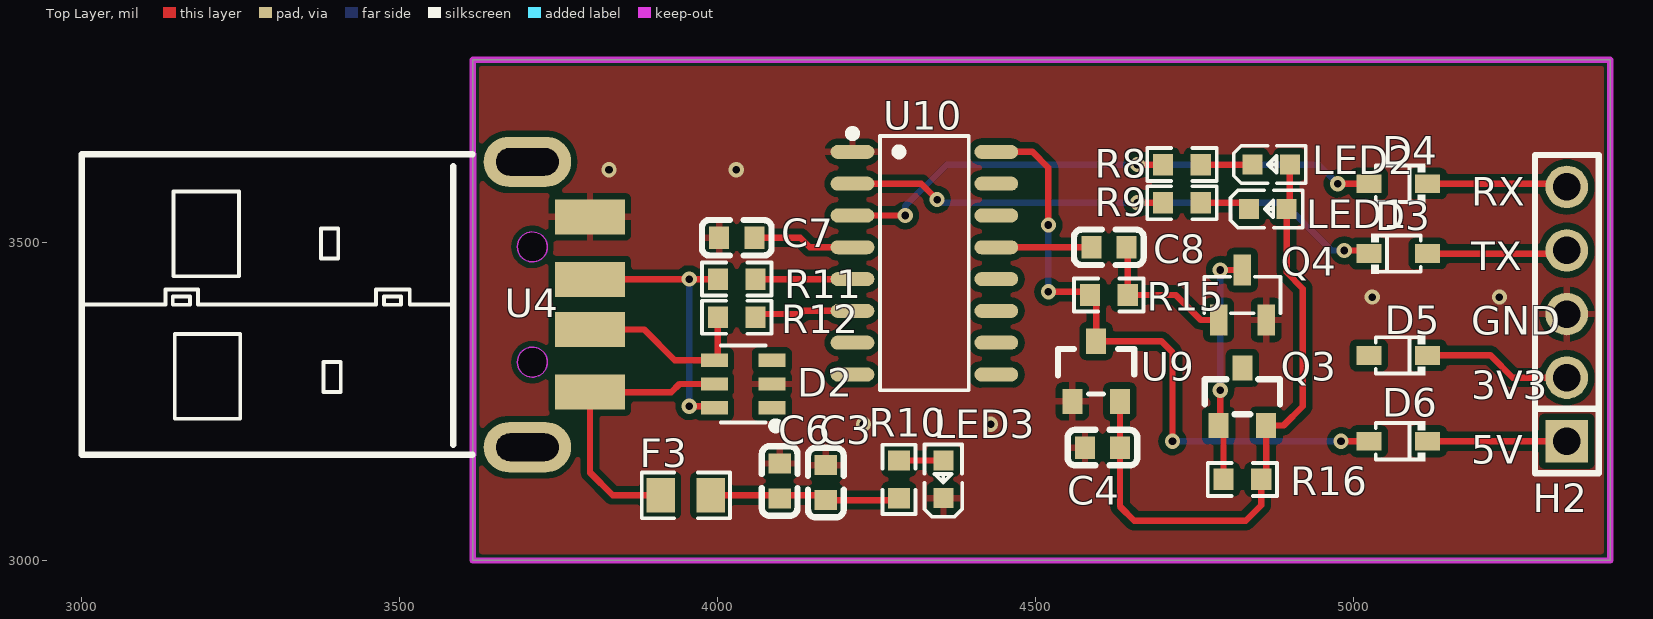
[diagram p0: Top Layer view]
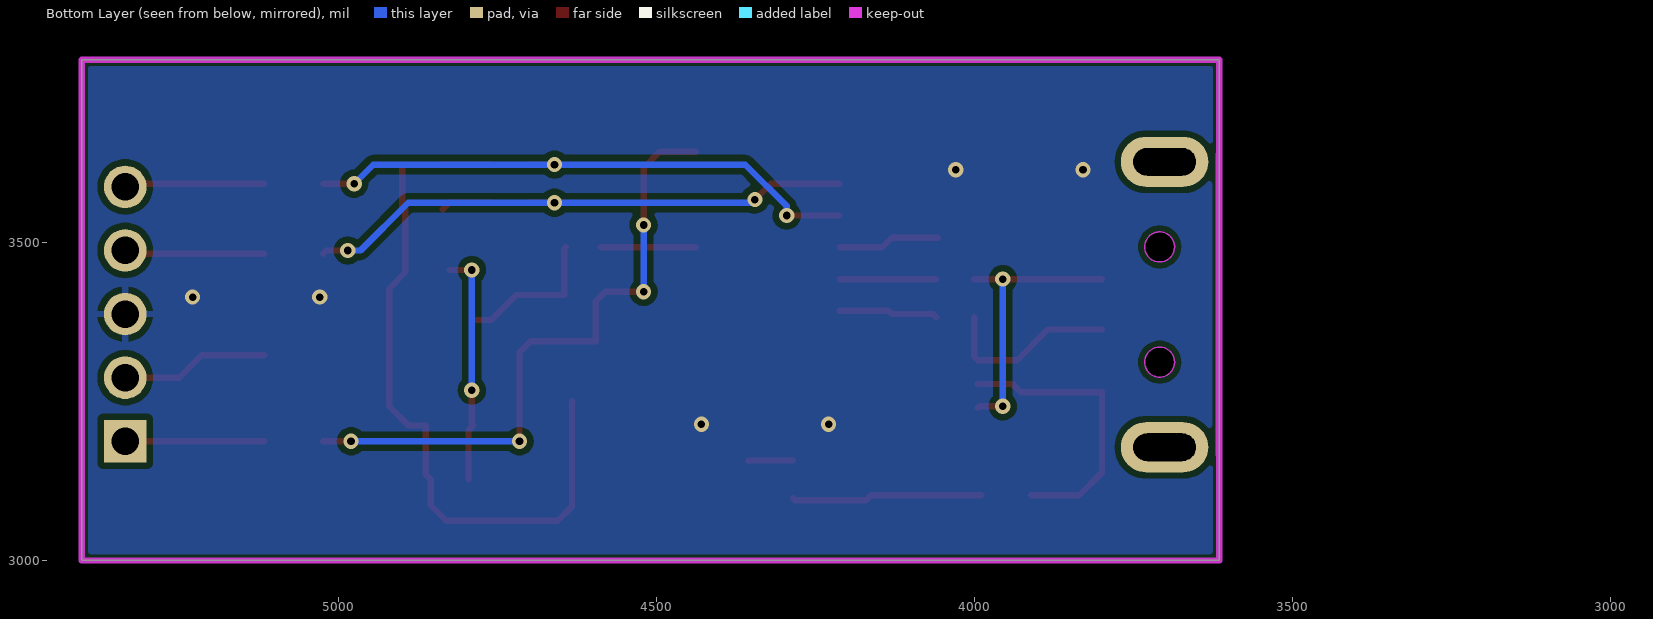
[diagram p1: Bottom Layer view, seen from below]
# Altium PCB MISC51088.pcbdoc
Units mil, origin at the board's own origin, x right, y up, seen from the top; angles counter-clockwise.
Board outline 1788.5 x 787.4 mil, 2 copper layers (Top Layer, Bottom Layer), stack 62.206 mil thick; 27 components, 24 nets, 82 pads, 20 vias.

## Layer stack, top to bottom
Top Solder Mask Layer: solder mask 0.394, Dk 3.3
Top Layer: signal copper 1.379
Dielectric1: surface 59.449, FR4, Dk 4.5
Bottom Layer: signal copper 1.378
Bottom Solder Mask Layer: solder mask 0.394, Dk 3.3

## Board outline
3615.01,3787.4 3615.01,3000 5403.51,3000 5403.51,3787.4

## Design rules (kind name [scope] priority, off if disabled: settings)
BoardOutlineClearance copperThickness2oz_1 [All] p2 off: genericclearance=7.99 ignorepadtopadclearanceinfootprint=FALSE except(0: Arc-SplitContinuation Track-SplitContinuation SMDPad-SplitContinuation THPad-SplitContinuation Via-SplitContinuation Fill-SplitContinuation Region-SplitContinuation Poly-SplitContinuation Text-SplitContinuation Hole-SplitContinuation; 5.98: Arc-CutoutEdge SMDPad-CutoutEdge THPad-CutoutEdge Via-CutoutEdge Fill-CutoutEdge Region-CutoutEdge Text-CutoutEdge; 6.93: Hole-OutlineEdge Hole-CutoutEdge; 10: Poly-OutlineEdge Poly-CutoutEdge; 11.81: Arc-OutlineEdge Track-OutlineEdge SMDPad-OutlineEdge THPad-OutlineEdge Via-OutlineEdge Fill-OutlineEdge Region-OutlineEdge Text-OutlineEdge Track-CutoutEdge)
BoardOutlineClearance Plane_innerPlane_1 [All] p4 off: genericclearance=4.02 ignorepadtopadclearanceinfootprint=FALSE except(0: Arc-SplitContinuation Track-SplitContinuation SMDPad-SplitContinuation THPad-SplitContinuation Via-SplitContinuation Fill-SplitContinuation Region-SplitContinuation Poly-SplitContinuation Text-SplitContinuation Hole-SplitContinuation; 6: SMDPad-CutoutEdge THPad-CutoutEdge Via-CutoutEdge Fill-CutoutEdge Region-CutoutEdge Text-CutoutEdge; 6.93: Hole-OutlineEdge Hole-CutoutEdge; 10: Poly-OutlineEdge Poly-CutoutEdge; 11.8: Arc-OutlineEdge Track-OutlineEdge SMDPad-OutlineEdge THPad-OutlineEdge Via-OutlineEdge Fill-OutlineEdge Region-OutlineEdge Text-OutlineEdge; 11.81: Arc-CutoutEdge Track-CutoutEdge)
BoardOutlineClearance Copper_copperRegion_1 [All] p6 off: genericclearance=4.02 ignorepadtopadclearanceinfootprint=FALSE except(0: Arc-SplitContinuation Track-SplitContinuation SMDPad-SplitContinuation THPad-SplitContinuation Via-SplitContinuation Fill-SplitContinuation Region-SplitContinuation Poly-SplitContinuation Text-SplitContinuation Hole-SplitContinuation; 6: SMDPad-CutoutEdge THPad-CutoutEdge Via-CutoutEdge Fill-CutoutEdge Region-CutoutEdge Text-CutoutEdge; 6.93: Hole-OutlineEdge Hole-CutoutEdge; 10: Poly-OutlineEdge Poly-CutoutEdge; 11.8: Arc-OutlineEdge Track-OutlineEdge SMDPad-OutlineEdge THPad-OutlineEdge Via-OutlineEdge Fill-OutlineEdge Region-OutlineEdge Text-OutlineEdge; 11.81: Arc-CutoutEdge Track-CutoutEdge)
BoardOutlineClearance Copper_copperRegion_copperThickness1oz_1 [All] p8 off: genericclearance=4.02 ignorepadtopadclearanceinfootprint=FALSE except(0: Arc-SplitContinuation Track-SplitContinuation SMDPad-SplitContinuation THPad-SplitContinuation Via-SplitContinuation Fill-SplitContinuation Region-SplitContinuation Poly-SplitContinuation Text-SplitContinuation Hole-SplitContinuation; 6: SMDPad-CutoutEdge THPad-CutoutEdge Via-CutoutEdge Fill-CutoutEdge Region-CutoutEdge Text-CutoutEdge; 6.93: Hole-OutlineEdge Hole-CutoutEdge; 10: Poly-OutlineEdge Poly-CutoutEdge; 11.8: Arc-OutlineEdge Track-OutlineEdge SMDPad-OutlineEdge THPad-OutlineEdge Via-OutlineEdge Fill-OutlineEdge Region-OutlineEdge Text-OutlineEdge; 11.81: Arc-CutoutEdge Track-CutoutEdge)
BoardOutlineClearance Copper_copperRegion_Copper_copperRegion_1 [All] p10 off: genericclearance=4.02 ignorepadtopadclearanceinfootprint=FALSE except(0: Arc-SplitContinuation Track-SplitContinuation SMDPad-SplitContinuation THPad-SplitContinuation Via-SplitContinuation Fill-SplitContinuation Region-SplitContinuation Poly-SplitContinuation Text-SplitContinuation Hole-SplitContinuation; 6: SMDPad-CutoutEdge THPad-CutoutEdge Via-CutoutEdge Fill-CutoutEdge Region-CutoutEdge Text-CutoutEdge; 6.93: Hole-OutlineEdge Hole-CutoutEdge; 10: Poly-OutlineEdge Poly-CutoutEdge; 11.8: Arc-OutlineEdge Track-OutlineEdge SMDPad-OutlineEdge THPad-OutlineEdge Via-OutlineEdge Fill-OutlineEdge Region-OutlineEdge Text-OutlineEdge; 11.81: Arc-CutoutEdge Track-CutoutEdge)
BoardOutlineClearance copperThickness1oz_1 [All] p12: genericclearance=4.02 ignorepadtopadclearanceinfootprint=FALSE except(0: Arc-SplitContinuation Track-SplitContinuation SMDPad-SplitContinuation THPad-SplitContinuation Via-SplitContinuation Fill-SplitContinuation Region-SplitContinuation Poly-SplitContinuation Text-SplitContinuation Hole-SplitContinuation; 6: SMDPad-CutoutEdge THPad-CutoutEdge Via-CutoutEdge Fill-CutoutEdge Region-CutoutEdge Text-CutoutEdge; 6.93: Hole-OutlineEdge Hole-CutoutEdge; 10: Poly-OutlineEdge Poly-CutoutEdge; 11.8: Arc-OutlineEdge Track-OutlineEdge SMDPad-OutlineEdge THPad-OutlineEdge Via-OutlineEdge Fill-OutlineEdge Region-OutlineEdge Text-OutlineEdge; 11.81: Arc-CutoutEdge Track-CutoutEdge)
Clearance copperThickness2oz [All] p1 off: gap=7.99 ignorepadtopadclearanceinfootprint=FALSE except(5.98: SMDPad-Track SMDPad-SMDPad THPad-Track SMDPad-THPad THPad-THPad Track-Via SMDPad-Via THPad-Via Via-Via Fill-Track Region-Track Fill-SMDPad Region-SMDPad Fill-THPad Region-THPad Fill-Via Region-Via Fill-Fill Fill-Region Region-Region Arc-Track Arc-SMDPad Arc-THPad Arc-Via Fill-Arc Region-Arc Arc-Arc Text-Track SMDPad-Text Text-THPad Text-Via Fill-Text Region-Text Arc-Text Text-Text; 6.93: Hole-Track Hole-SMDPad Hole-THPad Hole-Via Fill-Hole Region-Hole Hole-Arc Hole-Text; 10: Poly-Track Poly-SMDPad Poly-THPad Poly-Via Poly-Fill Poly-Region Poly-Poly Poly-Arc Poly-Text Poly-Hole)
Clearance Plane_innerPlane [All] p3 off: gap=4.02 ignorepadtopadclearanceinfootprint=FALSE except(5.98: SMDPad-Track SMDPad-SMDPad THPad-Track SMDPad-THPad THPad-THPad Track-Via SMDPad-Via THPad-Via Via-Via Fill-Track Region-Track Fill-SMDPad Region-SMDPad Fill-THPad Region-THPad Fill-Via Region-Via Fill-Fill Fill-Region Region-Region; 6: Arc-Track Arc-SMDPad Arc-THPad Arc-Via Fill-Arc Region-Arc Arc-Arc Text-Track SMDPad-Text Text-THPad Text-Via Fill-Text Region-Text Arc-Text Text-Text; 6.93: Hole-Track Hole-SMDPad Hole-THPad Hole-Via Fill-Hole Region-Hole Hole-Arc Hole-Text; 10: Poly-Track Poly-SMDPad Poly-THPad Poly-Via Poly-Fill Poly-Region Poly-Poly Poly-Arc Poly-Text Poly-Hole)
Clearance Copper_copperRegion [All] p5 off: gap=4.02 ignorepadtopadclearanceinfootprint=FALSE except(5.98: SMDPad-Track SMDPad-SMDPad THPad-Track SMDPad-THPad THPad-THPad Track-Via SMDPad-Via THPad-Via Via-Via Fill-Track Region-Track Fill-SMDPad Region-SMDPad Fill-THPad Region-THPad Fill-Via Region-Via Fill-Fill Fill-Region Region-Region; 6: Arc-Track Arc-SMDPad Arc-THPad Arc-Via Fill-Arc Region-Arc Arc-Arc Text-Track SMDPad-Text Text-THPad Text-Via Fill-Text Region-Text Arc-Text Text-Text; 6.93: Hole-Track Hole-SMDPad Hole-THPad Hole-Via Fill-Hole Region-Hole Hole-Arc Hole-Text; 10: Poly-Track Poly-SMDPad Poly-THPad Poly-Via Poly-Fill Poly-Region Poly-Poly Poly-Arc Poly-Text Poly-Hole)
Clearance Copper_copperRegion_copperThickness1oz [All] p7 off: gap=4.02 ignorepadtopadclearanceinfootprint=FALSE except(5.98: SMDPad-Track SMDPad-SMDPad THPad-Track SMDPad-THPad THPad-THPad Track-Via SMDPad-Via THPad-Via Via-Via Fill-Track Region-Track Fill-SMDPad Region-SMDPad Fill-THPad Region-THPad Fill-Via Region-Via Fill-Fill Fill-Region Region-Region; 6: Arc-Track Arc-SMDPad Arc-THPad Arc-Via Fill-Arc Region-Arc Arc-Arc Text-Track SMDPad-Text Text-THPad Text-Via Fill-Text Region-Text Arc-Text Text-Text; 6.93: Hole-Track Hole-SMDPad Hole-THPad Hole-Via Fill-Hole Region-Hole Hole-Arc Hole-Text; 10: Poly-Track Poly-SMDPad Poly-THPad Poly-Via Poly-Fill Poly-Region Poly-Poly Poly-Arc Poly-Text Poly-Hole)
Clearance Copper_copperRegion_Copper_copperRegion [All] p9 off: gap=4.02 ignorepadtopadclearanceinfootprint=FALSE except(5.98: SMDPad-Track SMDPad-SMDPad THPad-Track SMDPad-THPad THPad-THPad Track-Via SMDPad-Via THPad-Via Via-Via Fill-Track Region-Track Fill-SMDPad Region-SMDPad Fill-THPad Region-THPad Fill-Via Region-Via Fill-Fill Fill-Region Region-Region; 6: Arc-Track Arc-SMDPad Arc-THPad Arc-Via Fill-Arc Region-Arc Arc-Arc Text-Track SMDPad-Text Text-THPad Text-Via Fill-Text Region-Text Arc-Text Text-Text; 6.93: Hole-Track Hole-SMDPad Hole-THPad Hole-Via Fill-Hole Region-Hole Hole-Arc Hole-Text; 10: Poly-Track Poly-SMDPad Poly-THPad Poly-Via Poly-Fill Poly-Region Poly-Poly Poly-Arc Poly-Text Poly-Hole)
Clearance copperThickness1oz [All] p11: gap=4.02 ignorepadtopadclearanceinfootprint=FALSE except(5.98: SMDPad-Track SMDPad-SMDPad THPad-Track SMDPad-THPad THPad-THPad Track-Via SMDPad-Via THPad-Via Via-Via Fill-Track Region-Track Fill-SMDPad Region-SMDPad Fill-THPad Region-THPad Fill-Via Region-Via Fill-Fill Fill-Region Region-Region; 6: Arc-Track Arc-SMDPad Arc-THPad Arc-Via Fill-Arc Region-Arc Arc-Arc Text-Track SMDPad-Text Text-THPad Text-Via Fill-Text Region-Text Arc-Text Text-Text; 6.93: Hole-Track Hole-SMDPad Hole-THPad Hole-Via Fill-Hole Region-Hole Hole-Arc Hole-Text; 10: Poly-Track Poly-SMDPad Poly-THPad Poly-Via Poly-Fill Poly-Region Poly-Poly Poly-Arc Poly-Text Poly-Hole)
DiffPairsRouting differentialPair [All] p1: maxlimit=6 minlimit=6 mostfreqgap=6 toplayer_minwidth=5 toplayer_prefwidth=10 toplayer_maxwidth=100 toplayer_mingap=6 toplayer_prefgap=6 toplayer_maxgap=6 bottomlayer_minwidth=5 bottomlayer_prefwidth=10 bottomlayer_maxwidth=100 bottomlayer_mingap=6 bottomlayer_prefgap=6 bottomlayer_maxgap=6 maxuncoupledlength=10
HoleToHoleClearance otherClearance [All] p1: gap=11.81 allowstackedmicrovias=TRUE
Length netLength [All] p1: minlimit=0 maxlimit=0
PasteMaskExpansion pasteMaskExpansion [All] p1: expansion=0
PlaneConnect innerPlane [All] p1: planeconnectstyle=Relief reliefexpansion=20 reliefentries=4 reliefconductorwidth=10 reliefairgap=10
PolygonConnect copperRegion_copperThickness1oz [All] p1 off: connectstyle=Relief reliefconductorwidth=10 reliefentries=4 polygonreliefangle="90 Angle" airgapwidth=10 via.connectstyle=Relief via.reliefconductorwidth=10 via.reliefentries=4 via.polygonreliefangle="90 Angle" via.airgapwidth=10
PolygonConnect copperRegion_Copper_copperRegion [All] p2 off: connectstyle=Relief reliefconductorwidth=10 reliefentries=4 polygonreliefangle="90 Angle" airgapwidth=10 via.connectstyle=Relief via.reliefconductorwidth=10 via.reliefentries=4 via.polygonreliefangle="90 Angle" via.airgapwidth=10
PolygonConnect copperRegion [All] p3: connectstyle=Relief reliefconductorwidth=10 reliefentries=4 polygonreliefangle="90 Angle" airgapwidth=10 via.connectstyle=Relief via.reliefconductorwidth=10 via.reliefentries=4 via.polygonreliefangle="90 Angle" via.airgapwidth=10
RoutingVias viaSize [All] p1: holewidth=12.01 width=24.02 viastyle="Through Hole" minholewidth=11.81 minwidth=19.68 maxholewidth=248.03 maxwidth=393.7
SolderMaskExpansion solderMaskExpansion [IsVia] p1: expansion=-1000 istentingtop=TRUE
SolderMaskExpansion solderMaskExpansion [All] p2: expansion=2 istentingtop=FALSE
Width copperThickness2oz_2 [All] p1 off: maxlimit=100 minlimit=8 preferedwidth=10
Width copperThickness1oz_2 [All] p2: maxlimit=100 minlimit=5 preferedwidth=10

## Components (designator, comment, footprint, x,y, rotation, side; value= is the part's Value field where it differs from the comment)
C3 "100nF" C0603 4170.01,3122.4 r90 top
C4 "100nF" C0603 4605.01,3177.4 r0 top
C6 "100nF" C0603 4097.51,3124.9 r270 top
C7 "100nF" C0603 4030.01,3507.4 r180 top
C8 "10uF" C0603 4615.01,3492.4 r180 top
D2 "USBLC6-2SC6" SOT-23-6_L2.9-W1.6-P0.95-LS2.8-BL 4040.01,3277.4 r90 top
D3 "1N5819WS" SOD-323_L1.8-W1.3-LS2.5-RD 5070.01,3482.4 r0 top
D4 "1N5819WS" SOD-323_L1.8-W1.3-LS2.5-RD 5070.01,3592.4 r180 top
D5 "1N5819WS" SOD-323_L1.8-W1.3-LS2.5-RD 5070.01,3322.4 r180 top
D6 "1N5819WS" SOD-323_L1.8-W1.3-LS2.5-RD 5070.01,3187.4 r180 top
F3 "SMD0805-100-12" R0805 3950.01,3102.4 r0 top
H2 "PZ254V-11-05P" HDR-TH_5P-P2.54-V-M 5335.01,3387.4 r90 top
LED1 "MHT192DUGCT" LED0603-RD 4865.01,3552.4 r0 top
LED2 "LTST-C193KRKT-5A" LED0603-RD 4870.01,3622.4 r0 top
LED3 "MHT192DUGCT" LED0603-RD 4355.01,3127.4 r90 top
Q3 "AO3401A" SOT-23_L2.9-W1.3-P1.90-LS2.4-BR 4825.01,3257.4 r270 top
Q4 "S8050-J3Y" SOT-23-3_L2.9-W1.3-P0.95-LS2.4-BR-1 4825.01,3417.4 r270 top
R8 "1kΩ" R0603 4730.01,3622.4 r0 top
R9 "1kΩ" R0603 4730.01,3562.4 r0 top
R10 "10kΩ" R0603 4285.01,3127.4 r270 top
R11 "33kΩ" R0603 4030.01,3442.4 r0 top
R12 "33kΩ" R0603 4030.01,3382.4 r0 top
R15 "10kΩ" R0603 4615.01,3417.4 r180 top
R16 "10kΩ" R0603 4825.01,3127.4 r0 top
U4 "KH-USB180-AM-4P" USB-A-SMD_USB-A-1-TH 3750.01,3402.4 r180 top
U9 "XC6206-3.3V" SSOT-3_L2.9-W1.6-P0.95-LS2.8-BR 4595.01,3297.4 r270 top
U10 "CH340C" SOP-16_L10.0-W3.9-P1.27-LS6.0-BL 4325.01,3467.4 r270 top

## Footprints (in the part's own frame and the unit in brackets; to place one, negate y for a bottom-side part, rotate by r counter-clockwise, add the part's x,y. Pads: shape width x height; smd on the part's side, far side on the other; paste and mask are expansions set on the pad)
C0603 [mm]
  rect 0.8x0.9 smd: 1(-0.7,0) 2(0.7,0)
  silkscreen extent -1.39,-0.71 1.39,0.71
HDR-TH_5P-P2.54-V-M [mm]
  rect 1.7x1.7 hole 1.1: 1(-5.08,0)
  round 1.7 hole 1.1: 2(-2.54,0) 3(0,0) 4(2.54,0) 5(5.08,0)
  silkscreen extent -6.35,-1.27 6.35,1.27
LED0603-RD [mm]
  rect 0.8x0.8 smd: 1(-0.749,0) 2(0.749,0)
  silkscreen extent -1.49,-0.75 1.39,0.76
R0603 [mil]
  rect 31.75x34.02 smd paste-3937.01 mask+2: 1(-29.66,0) 2(29.66,0)
  silkscreen extent -55,-26 55,26
R0805 [mm]
  rect 1.133x1.377 smd paste-100 mask+0.051: 1(-1,0) 2(1,0)
  silkscreen extent -1.76,-0.92 1.76,0.92
SOD-323_L1.8-W1.3-LS2.5-RD [mm]
  rect 1x0.75 smd: 1(-1.173,0) 2(1.173,0)
  silkscreen extent -1.08,-0.8 0.9,0.8
SOP-16_L10.0-W3.9-P1.27-LS6.0-BL [mm]
  oval 0.56x1.745 smd: 1(-4.445,-2.872) 2(-3.175,-2.872) 3(-1.905,-2.872) 4(-0.635,-2.872) 5(0.635,-2.872) 6(1.905,-2.872) 7(3.175,-2.872) 8(4.445,-2.872) 9(4.445,2.872) 10(3.175,2.872) 11(1.905,2.872) 12(0.635,2.872) 13(-0.635,2.872) 14(-1.905,2.872) 15(-3.175,2.872) 16(-4.445,2.872)
  silkscreen extent -5.33,-3.02 5.08,1.77
SOT-23-3_L2.9-W1.3-P0.95-LS2.4-BR-1 [mm]
  rect 1.25x0.7 smd: 1(1,-0.95) 2(1,0.95) 3(-1,0)
  silkscreen extent -0.73,-1.53 0.73,1.53
SOT-23-6_L2.9-W1.6-P0.95-LS2.8-BL [mil]
  rect 20.95x42.2 smd: 1(-37.4,-45.24) 2(0,-45.24) 3(37.4,-45.24) 4(37.4,45.24) 5(0,45.24) 6(-37.4,45.24)
  silkscreen extent -72,-57 61,35
SOT-23_L2.9-W1.3-P1.90-LS2.4-BR [mm]
  rect 1x0.8 smd: 1(1.15,-0.95) 2(1.15,0.95) 3(-1.15,0)
  silkscreen extent -0.7,-1.5 0.7,1.5
SSOT-3_L2.9-W1.6-P0.95-LS2.8-BR [mm]
  rect 1x0.8 smd: 1(1.2,-0.95) 2(1.2,0.95) 3(-1.2,0)
  silkscreen extent -0.89,-1.52 0.9,1.52
USB-A-SMD_USB-A-1-TH [mm]
  rect 2.8x1.4 smd paste-100 mask+0.051: 1(-1.25,3.5) 2(-1.25,1) 3(-1.25,-1) 4(-1.25,-3.5)
  oval 3.5x2 hole 1.1 slot 2.5 at 0 deg: 5(1.25,5.7) 6(1.25,-5.7)
  Board Outline Layer circle w0.003: c1.05,2.3 r0.6
  Board Outline Layer circle w0.003: c1.05,-2.3 r0.6
  Board Outline Layer lines w0.254: 3.4,6 3.4,-6
  Board Outline Layer region: 0.45,2.3 0.509,2.56 0.676,2.769 0.916,2.885 1.183,2.885 1.424,2.769 1.59,2.56 1.65,2.3 1.65,2.3 1.59,2.04 1.424,1.831 1.183,1.715 0.916,1.715 0.676,1.831 0.509,2.04 0.45,2.3
  Board Outline Layer region: 0.45,2.3 0.459,2.404 0.486,2.505 0.53,2.6 0.59,2.686 0.664,2.76 0.75,2.82 0.845,2.864 0.946,2.891 1.05,2.9 1.154,2.891 1.255,2.864 1.35,2.82 1.436,2.76 1.51,2.686 1.57,2.6 1.614,2.505 1.641,2.404 1.65,2.3 1.641,2.196 1.614,2.095 1.57,2 1.51,1.914 1.436,1.84 1.35,1.78 1.255,1.736 1.154,1.709 1.05,1.7 0.946,1.709 0.845,1.736 0.75,1.78 0.664,1.84 0.59,1.914 0.53,2 0.486,2.095 0.459,2.196
  Board Outline Layer region: 0.45,-2.3 0.509,-2.04 0.676,-1.831 0.916,-1.715 1.183,-1.715 1.424,-1.831 1.59,-2.04 1.65,-2.3 1.65,-2.3 1.59,-2.56 1.424,-2.769 1.183,-2.885 0.916,-2.885 0.676,-2.769 0.509,-2.56 0.45,-2.3
  Board Outline Layer region: 0.45,-2.3 0.459,-2.196 0.486,-2.095 0.53,-2 0.59,-1.914 0.664,-1.84 0.75,-1.78 0.845,-1.736 0.946,-1.709 1.05,-1.7 1.154,-1.709 1.255,-1.736 1.35,-1.78 1.436,-1.84 1.51,-1.914 1.57,-2 1.614,-2.095 1.641,-2.196 1.65,-2.3 1.641,-2.404 1.614,-2.505 1.57,-2.6 1.51,-2.686 1.436,-2.76 1.35,-2.82 1.255,-2.864 1.154,-2.891 1.05,-2.9 0.946,-2.891 0.845,-2.864 0.75,-2.82 0.664,-2.76 0.59,-2.686 0.53,-2.6 0.486,-2.505 0.459,-2.404
  Multi-Layer board cut-out: 0.45,2.3 0.509,2.56 0.676,2.769 0.916,2.885 1.183,2.885 1.424,2.769 1.59,2.56 1.65,2.3 1.65,2.3 1.59,2.04 1.424,1.831 1.183,1.715 0.916,1.715 0.676,1.831 0.509,2.04 0.45,2.3
  Multi-Layer board cut-out: 0.45,-2.3 0.509,-2.04 0.676,-1.831 0.916,-1.715 1.183,-1.715 1.424,-1.831 1.59,-2.04 1.65,-2.3 1.65,-2.3 1.59,-2.56 1.424,-2.769 1.183,-2.885 0.916,-2.885 0.676,-2.769 0.509,-2.56 0.45,-2.3
  silkscreen extent 3.44,-6 19.05,6

## Via types
v1: diameter 24.02, hole 12, Top Layer to Bottom Layer, 20 vias

## Nets (pads, with @x,y where several pads share a name; then routed paths per layer and width w, separated by ;. In a path a pad name is that pad's centre, name@x,y a point inside that pad or via, vN(x,y) a via of type N, cw(c..) or ccw(c..) an arc to the next point about the centre after c; other vN are vias at no path point)
$1N4: D2.4 R12.1 U4.2 | length 285.4
  Top Layer w10: U4.2 3884.38,3363.03 3932.61,3314.8 D2.4 4000.35,3320.38 R12.1
$1N5: D2.5 F3.1 U4.1 | length 453.5
  Top Layer w10: F3.1 3835.01,3102.4 3799.22,3138.19 U4.1 3927.22,3264.61 3940.01,3277.4 D2.5
$1N7: R11.2 U10.5 | length 152.2
  Top Layer w10: R11.2 U10.5
$1N8: R12.2 U10.6 | length 156.4
  Top Layer w10: R12.2 4064.67,3387.4 4130.01,3387.4 4135.01,3392.4 U10.6
$1N10: C7.1 U10.4 | length 160.6
  Top Layer w10: C7.1 4130.01,3507.4 4145.01,3492.4 U10.4
$1N12: D2.6 R11.1 U4.3 | length 442
  Top Layer w10: U4.3 3799.86,3442.4 v1(3955.13,3442.4) R11.1 ; v1(3955.13,3242.4) 3992.37,3242.4 D2.6
  Bottom Layer w10: v1(3955.13,3242.4) v1(3955.13,3442.4)
$1N13: C3.1 C6.2 F3.2 R10.2 | length 300
  Top Layer w10: F3.2 4162.45,3102.4 C3.1 4282.11,3094.84 R10.2
$1N14: LED3.2 R10.1 | length 70.1
  Top Layer w10: R10.1 4354.83,3157.06 LED3.2
$1N20: C8.2 U10.13 | length 149.3
  Top Layer w10: U10.13 C8.2
$1N22: C8.1 Q4.1 R15.1 | length 235.1
  Top Layer w10: C8.1 4644.67,3490.3 R15.1 4720.01,3417.4 4759.38,3378.03 Q4.1
$1N25: Q3.1 Q4.3 R16.1 | length 368.6
  Top Layer w10: v1(4790.01,3267.4) 4790.01,3214.53 Q3.1 4795.35,3204.39 R16.1 ; v1(4790.01,3456.77) Q4.3
  Bottom Layer w10: v1(4790.01,3267.4) v1(4790.01,3456.77)
$1N27: C4.2 LED1.2 LED2.2 Q3.2 R16.2 U9.2 | length 998.1
  Top Layer w10: U9.2 4632.57,3250 C4.2 4632.57,3084.84 4655.01,3062.4 4830.01,3062.4 4854.67,3087.06 R16.2 4862.41,3135.14 Q3.2 4889.73,3212.13 4920.01,3242.4 4920.01,3427.4 4894.5,3452.91 LED1.2 4899.5,3557.41 LED2.2
$1N28: D6.1 H2.1 | length 218.8
  Top Layer w10: D6.1 H2.1
$1N30: D5.1 H2.2 | length 233.3
  Top Layer w10: D5.1 5215.01,3322.4 5250.01,3287.4 H2.2
$1N35: D4.1 H2.5 | length 220.9
  Top Layer w10: D4.1 5330.01,3592.4 H2.5
$1N36: D3.2 H2.4 | length 220.9
  Top Layer w10: D3.2 5330.01,3482.4 H2.4
$1N38: D4.2 R8.1 U10.3 | length 906.6
  Top Layer w10: U10.3 v1(4295.01,3542.4) ; v1(4660.01,3622.4) R8.1 ; v1(4975.01,3592.4) D4.2
  Bottom Layer w10: v1(4295.01,3542.4) 4295.01,3557.4 4360.01,3622.4 v1(4660.01,3622.4) 4945.01,3622.4 v1(4975.01,3592.4)
$1N39: LED2.1 R8.2 | length 80.8
  Top Layer w10: R8.2 LED2.1
$1N40: LED1.1 R9.2 | length 80
  Top Layer w10: R9.2 4825.52,3562.4 LED1.1
$1N44: D3.1 R9.1 U10.2 | length 897.8
  Top Layer w10: U10.2 4320.01,3592.4 v1(4345.01,3567.4) ; v1(4660.01,3562.4) R9.1 ; v1(4985.01,3487.4) 5018.85,3487.4 D3.1
  Bottom Layer w10: v1(4345.01,3567.4) 4350.01,3562.4 v1(4660.01,3562.4) 4890.01,3562.4 4965.01,3487.4 v1(4985.01,3487.4)
+3.3V: D5.2
+3V: Q3.3
+5V: D6.2 R15.2 U9.3 U10.16 | length 1007.4
  Top Layer w10: U10.16 4495.01,3642.4 4520.01,3617.4 v1(4520.01,3527.4) ; v1(4520.01,3422.4) 4580.35,3422.4 R15.2 4595.01,3407.74 U9.3 4697.77,3344.64 4715.01,3327.4 v1(4715.01,3187.4) ; v1(4980.01,3187.4) D6.2
  Bottom Layer w10: v1(4520.01,3422.4) v1(4520.01,3527.4) ; v1(4715.01,3187.4) v1(4980.01,3187.4)
GND: C3.2 C4.1 C6.1 C7.2 D2.2 H2.3 LED3.1 Q4.2 U4.4 U9.1 U10.1
  other v1: 4229.11,3214.1 4429.11,3214.1 5029.11,3414.1 5229.11,3414.1 3829.11,3614.1 4029.11,3614.1
pads on no net: D2.1 D2.3 U4.5 U4.6 U10.7 U10.8 U10.9 U10.10 U10.11 U10.12 U10.14 U10.15

## Polygon pours and split planes (outlines as drawn)
GND on Top Layer (solid, remove dead copper, pour order 0): 3615.01,3787.4 3615.01,3000 5583.51,3000 5583.51,3787.4
GND on Bottom Layer (solid, remove dead copper, pour order 2): 3615.01,3777.73 3615.01,3000 5583.51,3000 5583.51,3777.73

## Keep-outs
Board Outline Layer:
  the board outline again, w10

## Silkscreen, mask and mechanical layers (free items; w line width, h text height)
Top Silkscreen Layer:
  text "RX" at 5185.01,3557.4 h45
  text "TX" at 5185.01,3456.15 h45
  text "GND" at 5185.01,3354.9 h45
  text "3V3" at 5185.01,3253.65 h45
  text "5V" at 5185.01,3152.4 h45